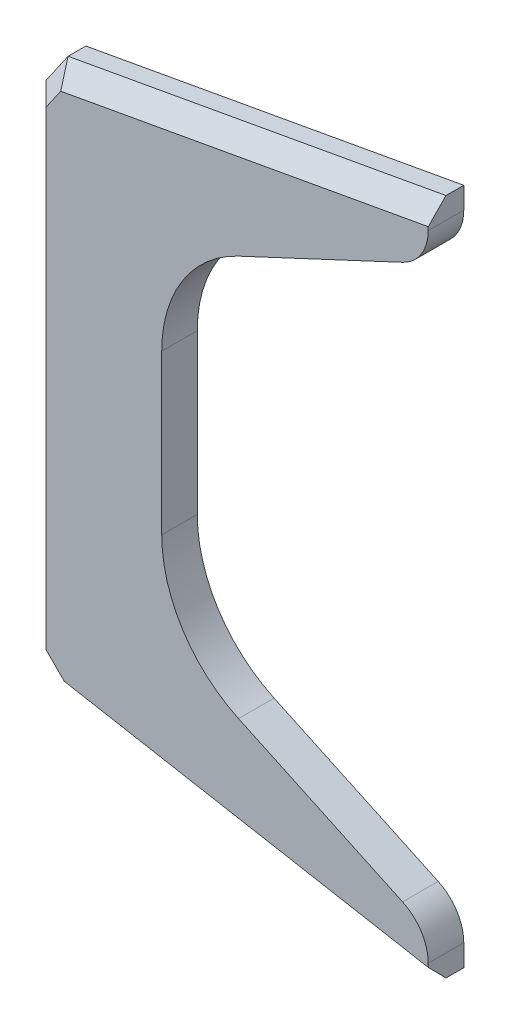
from build123d import *
from OCP.BRepFilletAPI import BRepFilletAPI_MakeChamfer

# Parameters (mm, degrees)
BOSS_EXTRUDE1_DEPTH = 16
CHAMFER1_SIZE       = 10
CHAMFER1_SIZE2      = 12.4055197
CHAMFER2_SIZE       = 8


with BuildPart() as part:
    # Sketch1 → Boss-Extrude1 (new body)
    with BuildSketch(Plane.XY):
        with BuildLine():
            Line((0, -120), (0, 120))
            Line((0, 120), (180, 152.55))
            Line((180, 152.55), (180, 142.864097444))
            ThreePointArc((180, 142.864097444), (176.872536286, 132.125497941), (168.468248072, 124.745356467))
            Line((168.468248072, 124.745356467), (94.595255785, 90.218960551))
            ThreePointArc((94.595255785, 90.218960551), (69.382391143, 68.078536128), (60, 35.862737619))
            Line((60, 35.862737619), (60, -35.762737619))
            ThreePointArc((60, -35.762737619), (69.382391143, -67.978536128), (94.595255785, -90.118960551))
            Line((94.595255785, -90.118960551), (168.468248072, -124.645356467))
            ThreePointArc((168.468248072, -124.645356467), (176.872536286, -132.025497941), (180, -142.764097444))
            Line((180, -142.764097444), (180, -152.55))
            Line((180, -152.55), (0, -120))
        make_face()
    extrude(amount=BOSS_EXTRUDE1_DEPTH)

    # Chamfer1: one chamfer whose edges measure the first distance from different faces: ONE call of the kernel's chamfer builder (chamfer() names one face for all edges)
    chamfer1_edges_1 = [part.edges().sort_by_distance(p)[0] for p in [
        (0, -120, 8),
    ]]
    chamfer1_side_1 = [part.faces().sort_by_distance(p)[0] for p in [
        (0, 0, 8),
    ]]
    chamfer1_edges_2 = [part.edges().sort_by_distance(p)[0] for p in [
        (0, 120, 8),
    ]]
    chamfer1_side_2 = [part.faces().sort_by_distance(p)[0] for p in [
        (90, 136.275, 8),
    ]]
    chamfer1 = BRepFilletAPI_MakeChamfer(part.part.solid().wrapped)
    for e in chamfer1_edges_1:
        chamfer1.Add(CHAMFER1_SIZE, CHAMFER1_SIZE2, e.wrapped, chamfer1_side_1[0].wrapped)  # the first distance lies on this face
    for e in chamfer1_edges_2:
        chamfer1.Add(CHAMFER1_SIZE, CHAMFER1_SIZE2, e.wrapped, chamfer1_side_2[0].wrapped)  # the first distance lies on this face
    add(Compound.cast(chamfer1.Shape()), mode=Mode.REPLACE)

    # Chamfer2
    chamfer2_edges = [part.edges().sort_by_distance(p)[0] for p in [
        (0, -1.20275985, 16),
        (96.103763988, -137.378763988, 16),
        (6.103763988, -116.103763988, 16),
        (4.920200149, 114.686976343, 16),
        (94.920200149, 137.164736194, 16),
    ]]
    chamfer(chamfer2_edges, length=CHAMFER2_SIZE)


solid = part.part
